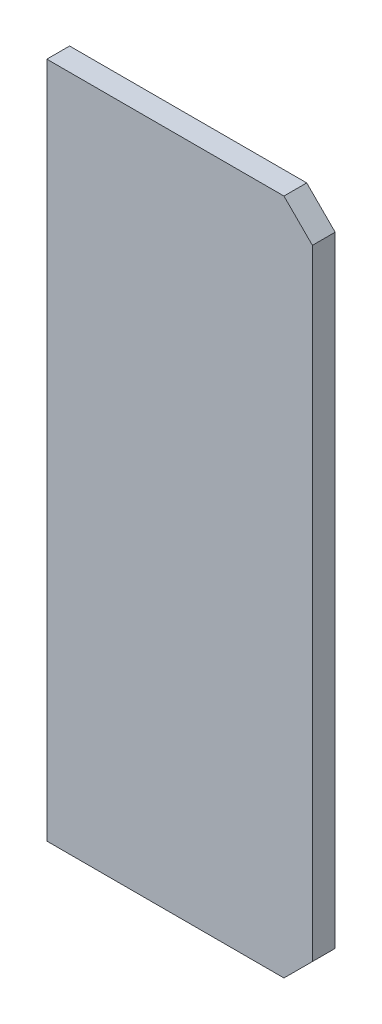
SolidWorks part; units mm, degrees
material "Q235"
ref_plane "Front Plane" through (0, 0, 0) normal (0, 0, 1) x (1, 0, 0)
ref_plane "Top Plane" through (0, 0, 0) normal (0, 1, 0) x (1, 0, 0)
ref_plane "Right Plane" through (0, 0, 0) normal (1, 0, 0) x (0, 0, -1)
sketch "Sketch1" plane through (0, 0, 0) normal (0, 0, 1) x (1, 0, 0)
  line L1 (0, 0) -> (140, 0)
  line L2 (0, 0) -> (0, 357)
  line L3 (0, 357) -> (140, 357)
  line L4 (140, 0) -> (140, 357)
  dimension "D1" = 140
  dimension "D2" = 357
extrude "Boss-Extrude1" add sketch "Sketch1" along normal blind 12
chamfer "Chamfer2" distance 15 angle 45 2 edges at (140, 0, 6) (140, 357, 6)
